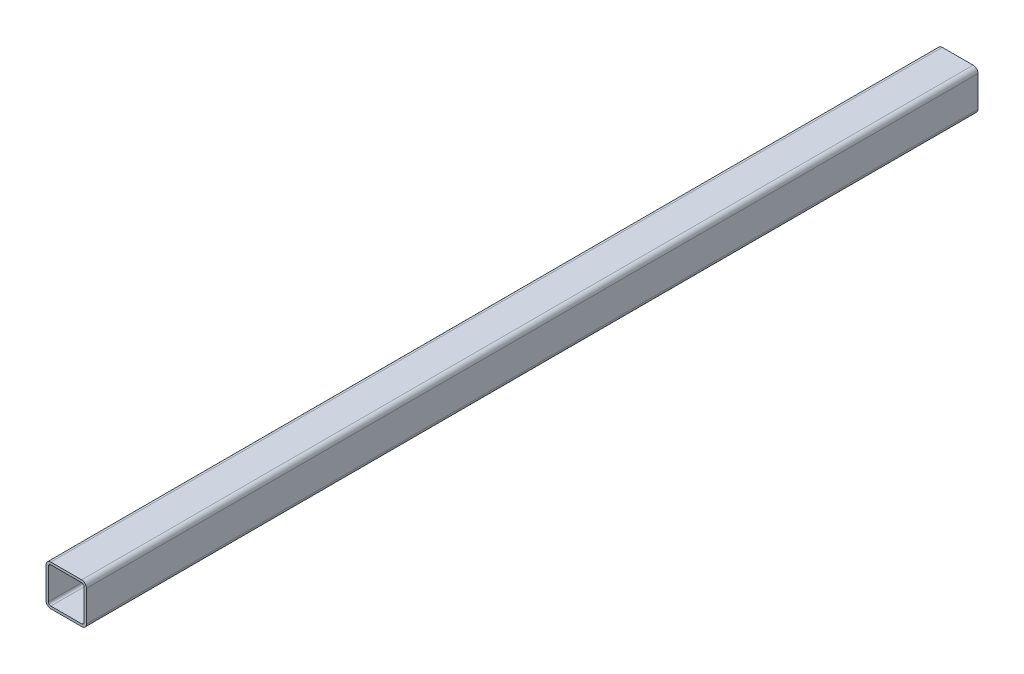
from build123d import *

# Parameters (mm, degrees)
GB_6728_1986_050_X_50_X_3_1_DEPTH = 1100


with BuildPart() as part:
    # Sketch1 → Gb／6728-1986方形空心型钢 050 X 50 X 3(1) (new body)
    with BuildSketch(Plane(origin=(0, 0, 0), x_dir=(-1, 0, 0), z_dir=(0, 0, -1))):
        with BuildLine():
            Line((-19, -25), (19, -25))
            ThreePointArc((19, -25), (23.242640687, -23.242640687), (25, -19))
            Line((25, -19), (25, 19))
            ThreePointArc((25, 19), (23.242640687, 23.242640687), (19, 25))
            Line((19, 25), (-19, 25))
            ThreePointArc((-19, 25), (-23.242640687, 23.242640687), (-25, 19))
            Line((-25, 19), (-25, -19))
            ThreePointArc((-25, -19), (-23.242640687, -23.242640687), (-19, -25))
        make_face()
        with BuildLine():
            Line((-19, -22), (19, -22))
            ThreePointArc((19, -22), (21.121320344, -21.121320344), (22, -19))
            Line((22, -19), (22, 19))
            ThreePointArc((22, 19), (21.121320344, 21.121320344), (19, 22))
            Line((19, 22), (-19, 22))
            ThreePointArc((-19, 22), (-21.121320344, 21.121320344), (-22, 19))
            Line((-22, 19), (-22, -19))
            ThreePointArc((-22, -19), (-21.121320344, -21.121320344), (-19, -22))
        make_face(mode=Mode.SUBTRACT)
    extrude(amount=GB_6728_1986_050_X_50_X_3_1_DEPTH)


solid = part.part
